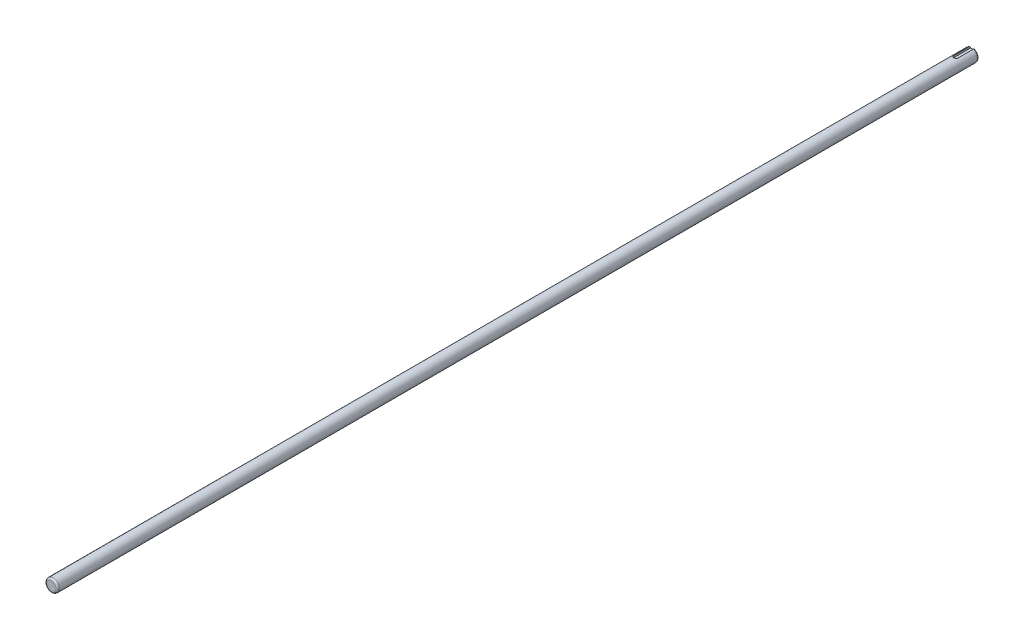
SolidWorks part; units mm, degrees
ref_plane "前视基准面" through (0, 0, 0) normal (0, 0, 1) x (1, 0, 0)
ref_plane "上视基准面" through (0, 0, 0) normal (0, 1, 0) x (1, 0, 0)
ref_plane "右视基准面" through (0, 0, 0) normal (1, 0, 0) x (0, 0, -1)
sketch "草图1" plane through (0, 0, 0) normal (0, 0, 1) x (1, 0, 0)
  circle A0 centre (0, 0) radius 7.5
  dimension "D1" = 15
extrude "拉伸1" add sketch "草图1" along normal mid plane 1090
fillet "圆角1" radius 2 2 edges at (7.5, 0, -545) (7.5, 0, 545)
sketch "草图2" plane through (0, 0, -545) normal (0, 0, -1) x (-1, 0, 0)
  line L1 (-2.5, 5) -> (-2.5, 11.7696)
  line L2 (-2.5, 11.7696) -> (2.5, 11.7696)
  line L3 (2.5, 11.7696) -> (2.5, 5)
  line L5 (-2.5, 5) -> (2.5, 5)
  dimension "D1" = 5
  dimension "D3" = 5
extrude "拉伸2" cut sketch "草图2" against normal blind 20
sketch "草图3" plane through (0, 5, 0) normal (0, 1, 0) x (1, 0, 0)
  line L0 (2.5, 525) -> (-2.5, 525) construction
  circle A0 centre (0, 525) radius 2.5
extrude "拉伸3" cut sketch "草图3" along normal through all
